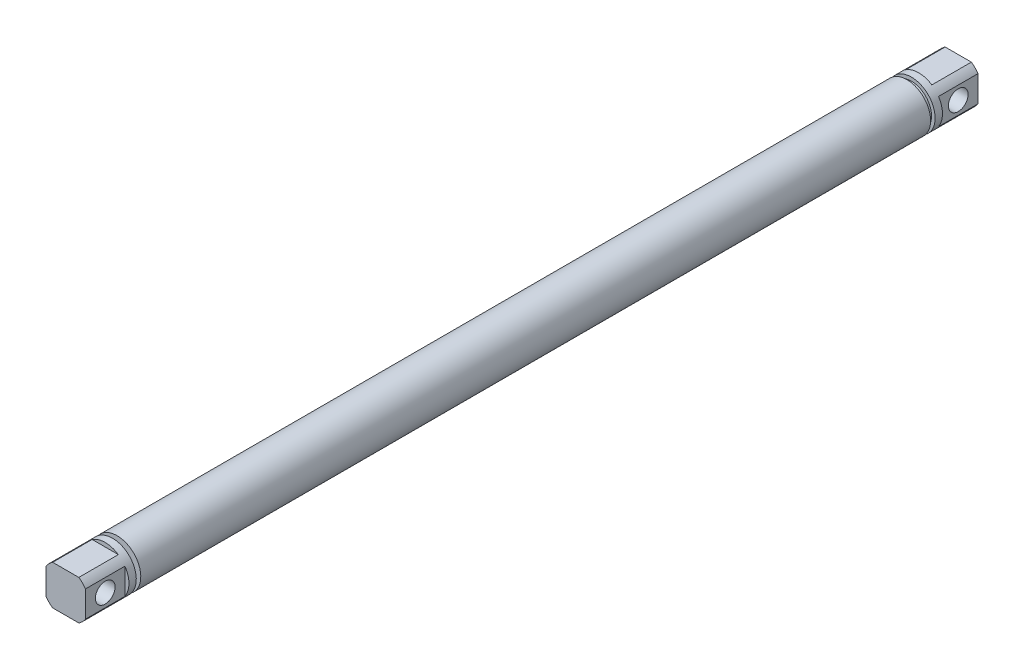
SolidWorks part; units mm, degrees
ref_plane "前视基准面" through (0, 0, 0) normal (0, 0, 1) x (1, 0, 0)
ref_plane "上视基准面" through (0, 0, 0) normal (0, 1, 0) x (1, 0, 0)
ref_plane "右视基准面" through (0, 0, 0) normal (1, 0, 0) x (0, 0, -1)
sketch "草图1" plane through (0, 0, 0) normal (0, 0, 1) x (1, 0, 0)
  circle A0 centre (0, 0) radius 6
  dimension "D1" = 12
extrude "凸台-拉伸1" add sketch "草图1" along normal mid plane 226
sketch "草图2" plane through (0, 0, 0) normal (1, 0, 0) x (0, 0, -1)
  line L0 (0, 0) -> (113, 0) construction
  line L1 (113, -6) -> (113, 6) construction
  line L2 (113, 6) -> (-113, 6) construction
  line L3 (101.14, 6) -> (100, 6)
  line L4 (101.14, 6) -> (101.14, 5.1)
  line L5 (101.14, 5.1) -> (100, 5.1)
  line L6 (100, 6) -> (100, 5.1)
  line L7 (0, 0) -> (0, 6) construction
  line L8 (-100, 6) -> (-101.14, 6)
  line L9 (-100, 6) -> (-100, 4.3457)
  line L10 (-100, 4.3457) -> (-101.14, 4.3457)
  line L11 (-101.14, 6) -> (-101.14, 4.3457)
  point P15 (0, 6)
  point P17 (0, 6)
  dimension "D1" = 1.14
  dimension "D2" = 200
  dimension "D3" = 5.1
revolve "切除-旋转1" cut sketch "草图2" angle 360 about L0
sketch "草图3" plane through (0, 0, -113) normal (0, 0, -1) x (-1, 0, 0)
  line L4 (-5, 3.3166) -> (-5, -3.3166)
  line L9 (5, 3.3166) -> (5, -3.3166)
  line L10 (0, 0) -> (0, 6) construction
  line L11 (-3.3166, 5) -> (3.3166, 5)
  line L12 (3.3166, -5) -> (-3.3166, -5)
  line L13 (0, 0) -> (6, 0) construction
  arc A0 (-5, 3.3166) -> (-5, -3.3166) centre (0, 0) ccw
  circle A1 centre (0, 0) radius 6 construction
  arc A2 (-3.3166, -5) -> (3.3166, -5) centre (0, 0) ccw
  arc A3 (5, -3.3166) -> (5, 3.3166) centre (0, 0) ccw
  arc A4 (3.3166, 5) -> (-3.3166, 5) centre (0, 0) ccw
  dimension "D1" = 10
  dimension "D2" = 10
extrude "切除-拉伸1" cut sketch "草图3" against normal blind 10
hole_wizard "M6 螺纹孔1" positions "草图4" profile "草图5" tap size "M6" standard "GB" end condition up to next
sketch "草图4" plane through (-5, 0, 0) normal (-1, 0, 0) x (0, 0, 1)
  line L0 (-113, 0) -> (-108, 0) construction
  line L1 (-113, 3.3166) -> (-113, -3.3166) construction
  point P0 (-108, 0)
  point P9 (0, 0)
  dimension "D1" = 5
sketch "草图5" plane through (-5, 0, -108) normal (0, 1, 0) x (0, 0, 1)
  line L0 (0, 0) -> (0, 10.001)
  line L1 (0, 10.001) -> (2.5, 10.001)
  line L2 (2.5, 10.001) -> (2.5, 0)
  line L5 (2.5, 0) -> (0, 0)
  line L11 (0, -6.35) -> (0, 107.95) construction
  dimension "通孔螺纹孔钻头直径" = 5
  dimension "通孔螺纹孔钻头深度" = 10.001
cosmetic thread "孔螺蚊线1" parameters "D2"=6
mirror "镜向1" about plane through (0, 0, 0) normal (0, 0, 1) of "M6 螺纹孔1", "切除-拉伸1"
